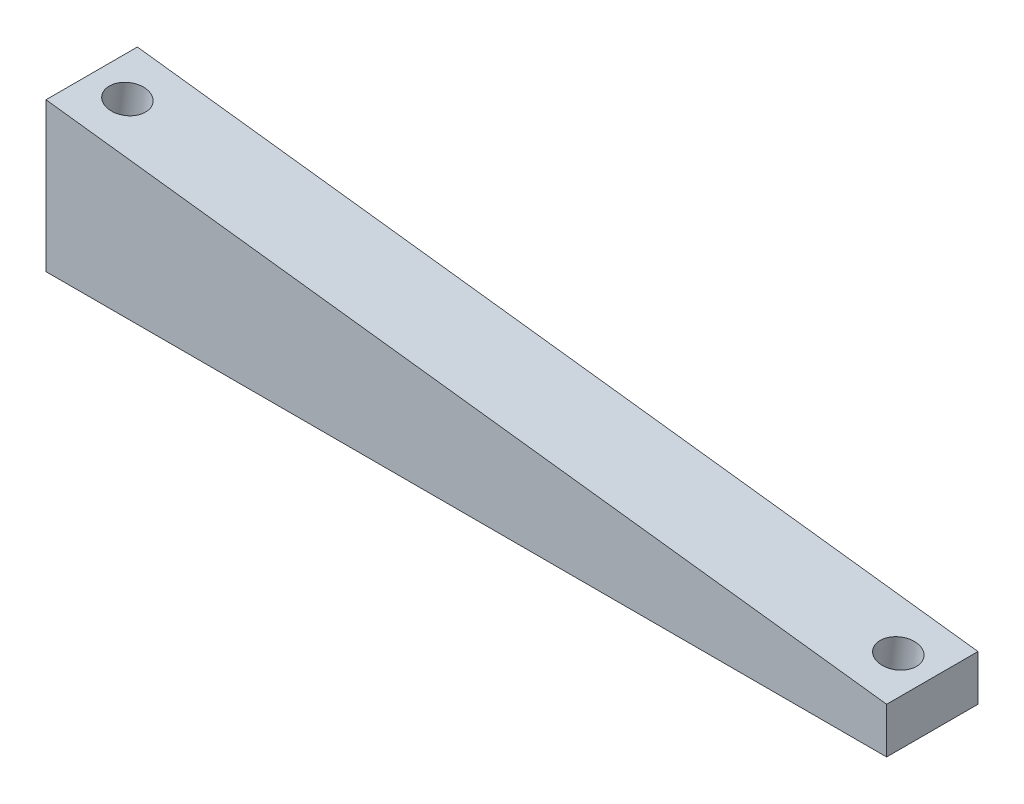
from build123d import *

# Parameters (mm, degrees)
BOSS_EXTRUDE1_DEPTH = 20
SKETCH2_R           = 4
CUT_EXTRUDE1_DEPTH  = 15
LPATTERN1_COUNT     = 2
LPATTERN1_PITCH     = 170


with BuildPart() as part:
    # Sketch1 → Boss-Extrude1 (new body)
    with BuildSketch(Plane.XY):
        Polygon((0, 0), (184, 0), (184, 10), (0, 32.592359206), align=None)
    extrude(amount=BOSS_EXTRUDE1_DEPTH)

    # Sketch2 → Cut-Extrude1 (cut)
    with BuildSketch(Plane(origin=(3.942402661, 32.108293027, 0), x_dir=(0.9925461516413229, -0.12186934340514068, 0), z_dir=(0.12186934340514069, 0.992546151641323, 0))):
        with Locations(Location((173.909798468, -10, 0), (0, 0, 180))):
            Circle(SKETCH2_R)
    cut_extrude1 = extrude(amount=-CUT_EXTRUDE1_DEPTH, mode=Mode.SUBTRACT)

    # LPattern1: Cut-Extrude1 ×2
    with Locations(*[Vector(-0.9925461516413229, 0.12186934340514068, 0) * (i * LPATTERN1_PITCH) for i in range(1, LPATTERN1_COUNT)]):
        add(cut_extrude1, mode=Mode.SUBTRACT)


solid = part.part
